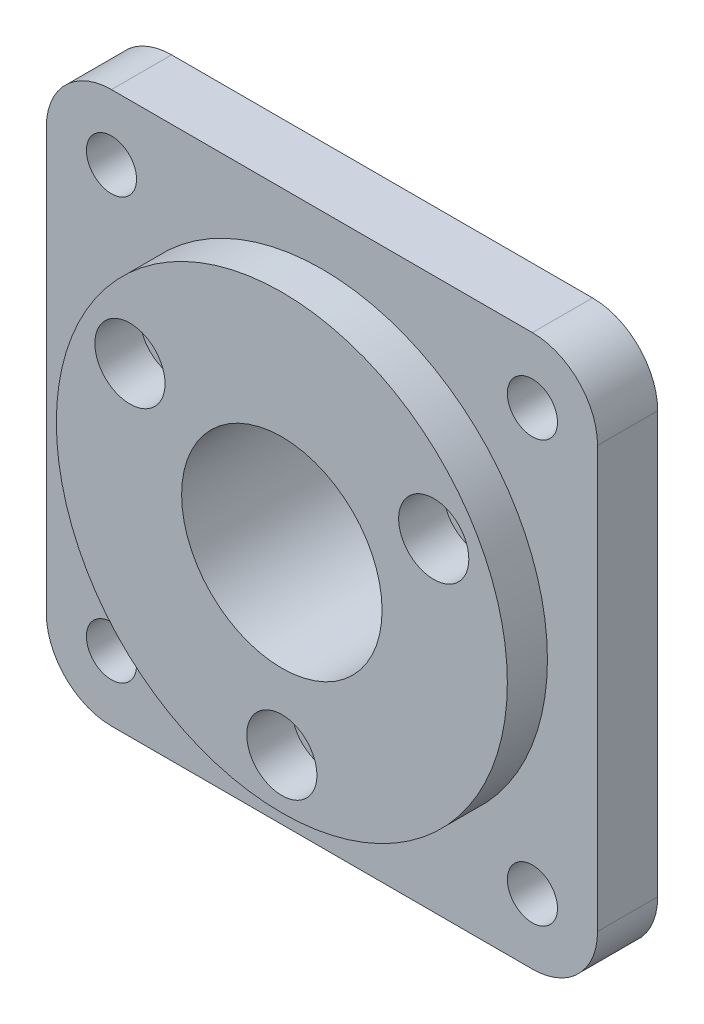
from build123d import *

# Parameters (mm, degrees)
BOSS_EXTRUDE1_DEPTH = 12
SKETCH2_R           = 5
CUT_EXTRUDE1_DEPTH  = 50
SKETCH3_R           = 45
BOSS_EXTRUDE2_DEPTH = 8
SKETCH4_R           = 23.5
BOSS_EXTRUDE3_DEPTH = 9.8
SKETCH6_R           = 20
CUT_EXTRUDE2_DEPTH  = 80
SKETCH7_R           = 7
CUT_EXTRUDE3_DEPTH  = 9
SKETCH8_R           = 4.5
CUT_EXTRUDE4_DEPTH  = 801
CIRPATTERN1_COUNT   = 3


with BuildPart() as part:
    # Sketch1 → Boss-Extrude1 (new body)
    with BuildSketch(Plane.XY):
        with BuildLine():
            Line((-42, -55), (42, -55))
            ThreePointArc((42, -55), (51.192388155, -51.192388155), (55, -42))
            Line((55, -42), (55, 42))
            ThreePointArc((55, 42), (51.192388155, 51.192388155), (42, 55))
            Line((42, 55), (-42, 55))
            ThreePointArc((-42, 55), (-51.192388155, 51.192388155), (-55, 42))
            Line((-55, 42), (-55, -42))
            ThreePointArc((-55, -42), (-51.192388155, -51.192388155), (-42, -55))
        make_face()
    extrude(amount=BOSS_EXTRUDE1_DEPTH)

    # Sketch2 → Cut-Extrude1 (cut)
    with BuildSketch(Plane.XY.offset(12)):
        with Locations((42, 42)):
            Circle(SKETCH2_R)
        with Locations((42, -42)):
            Circle(SKETCH2_R)
        with Locations((-42, -42)):
            Circle(SKETCH2_R)
        with Locations((-42, 42)):
            Circle(SKETCH2_R)
    extrude(amount=-CUT_EXTRUDE1_DEPTH, mode=Mode.SUBTRACT)

    # Sketch3 → Boss-Extrude2 (add)
    with BuildSketch(Plane.XY.offset(12)):
        Circle(SKETCH3_R)
    extrude(amount=BOSS_EXTRUDE2_DEPTH)

    # Sketch4 → Boss-Extrude3 (add)
    with BuildSketch(Plane(origin=(0, 0, 0), x_dir=(-1, 0, 0), z_dir=(0, 0, -1))):
        with Locations(Location((0, 0, 0), (0, 0, 180))):
            Circle(SKETCH4_R)
    extrude(amount=BOSS_EXTRUDE3_DEPTH)

    # Sketch6 → Cut-Extrude2 (cut)
    with BuildSketch(Plane(origin=(0, 0, -9.8), x_dir=(-1, 0, 0), z_dir=(0, 0, -1))):
        Circle(SKETCH6_R)
    extrude(amount=-CUT_EXTRUDE2_DEPTH, mode=Mode.SUBTRACT)

    # Sketch7 → Cut-Extrude3 (cut)
    with BuildSketch(Plane.XY.offset(20)):
        with Locations((0, -35)):
            Circle(SKETCH7_R)
    cut_extrude3 = extrude(amount=-CUT_EXTRUDE3_DEPTH, mode=Mode.SUBTRACT)

    # Sketch8 → Cut-Extrude4 (cut)
    with BuildSketch(Plane.XY.offset(11)):
        with Locations((0, -35)):
            Circle(SKETCH8_R)
    cut_extrude4 = extrude(amount=-CUT_EXTRUDE4_DEPTH, mode=Mode.SUBTRACT)

    # CirPattern1: Cut-Extrude3, Cut-Extrude4 ×3 about axis
    cirpattern1_axis = Axis((0, 0, 0), (0, 0, 1))
    add([cut_extrude3.rotate(cirpattern1_axis, i * 360 / CIRPATTERN1_COUNT) for i in range(1, CIRPATTERN1_COUNT)], mode=Mode.SUBTRACT)
    add([cut_extrude4.rotate(cirpattern1_axis, i * 360 / CIRPATTERN1_COUNT) for i in range(1, CIRPATTERN1_COUNT)], mode=Mode.SUBTRACT)


solid = part.part
